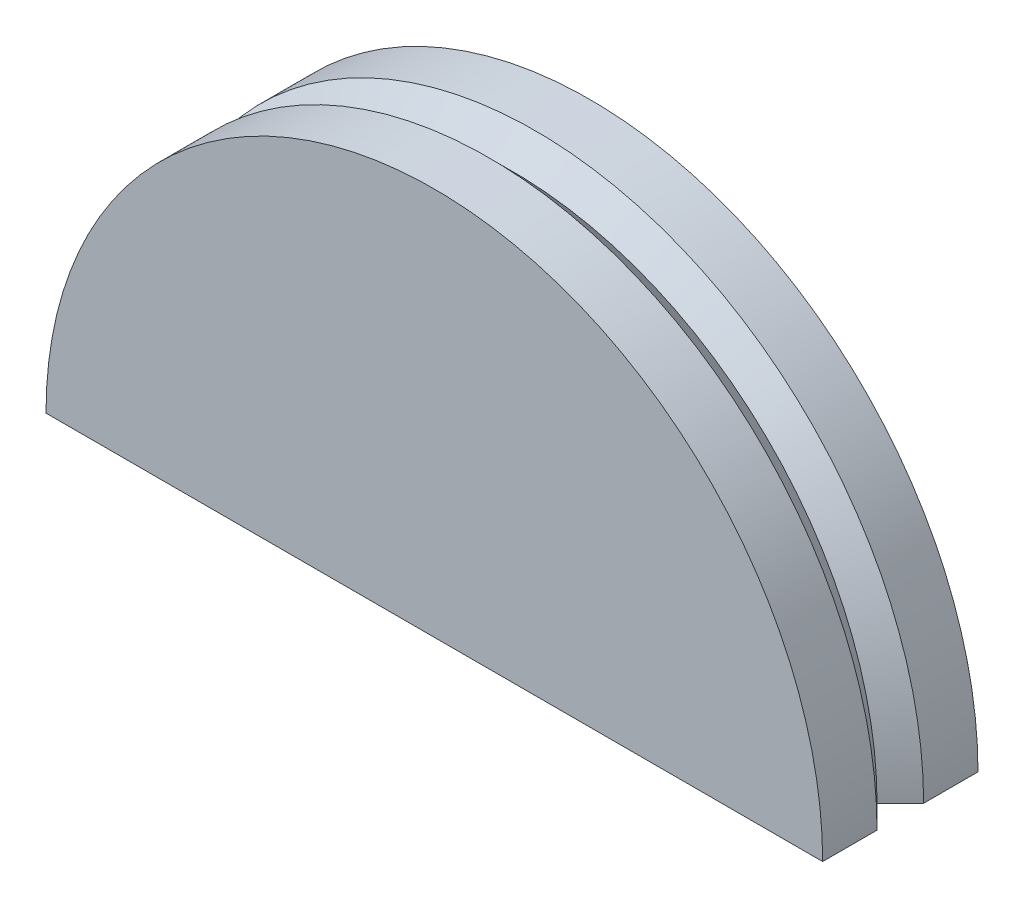
SolidWorks part; units mm, degrees
material "PBT general purpose"
ref_plane "Front Plane" through (0, 0, 0) normal (0, 0, 1) x (1, 0, 0)
ref_plane "Top Plane" through (0, 0, 0) normal (0, 1, 0) x (1, 0, 0)
ref_plane "Right Plane" through (0, 0, 0) normal (1, 0, 0) x (0, 0, -1)
sketch "Sketch1" plane through (0, 0, 0) normal (0, 0, 1) x (1, 0, 0)
  line L0 (-23.7452, -21.4683) -> (26.2548, -21.4683)
  arc A0 (26.2548, -21.4683) -> (-23.7452, -21.4683) centre (1.2548, -21.4683) ccw
extrude "Boss-Extrude1" add sketch "Sketch1" along normal blind 10
sketch "Sketch2" plane through (0, -21.4683, 0) normal (0, -1, 0) x (1, 0, 0)
  line L0 (26.2548, 5) -> (26.2548, 6.5)
  line L1 (26.2548, 10) -> (26.2548, 0) construction
  line L2 (26.2548, 5) -> (26.2548, 3.5)
  line L3 (26.2548, 6.5) -> (24.7548, 5)
  line L4 (24.7548, 5) -> (26.2548, 3.5)
ref_plane "Plane1" through (0, 0, 5) normal (0, 0, 1) x (1, 0, 0)
sketch "Sketch4" plane through (0, 0, 5) normal (0, 0, 1) x (1, 0, 0)
  line L0 (-23.7452, -21.4683) -> (26.2548, -21.4683) construction
  arc A0 (26.2548, -21.4683) -> (-23.7452, -21.4683) centre (1.2548, -21.4683) ccw
sweep "Cut-Sweep1" cut profiles "Sketch2" path "Sketch4"
